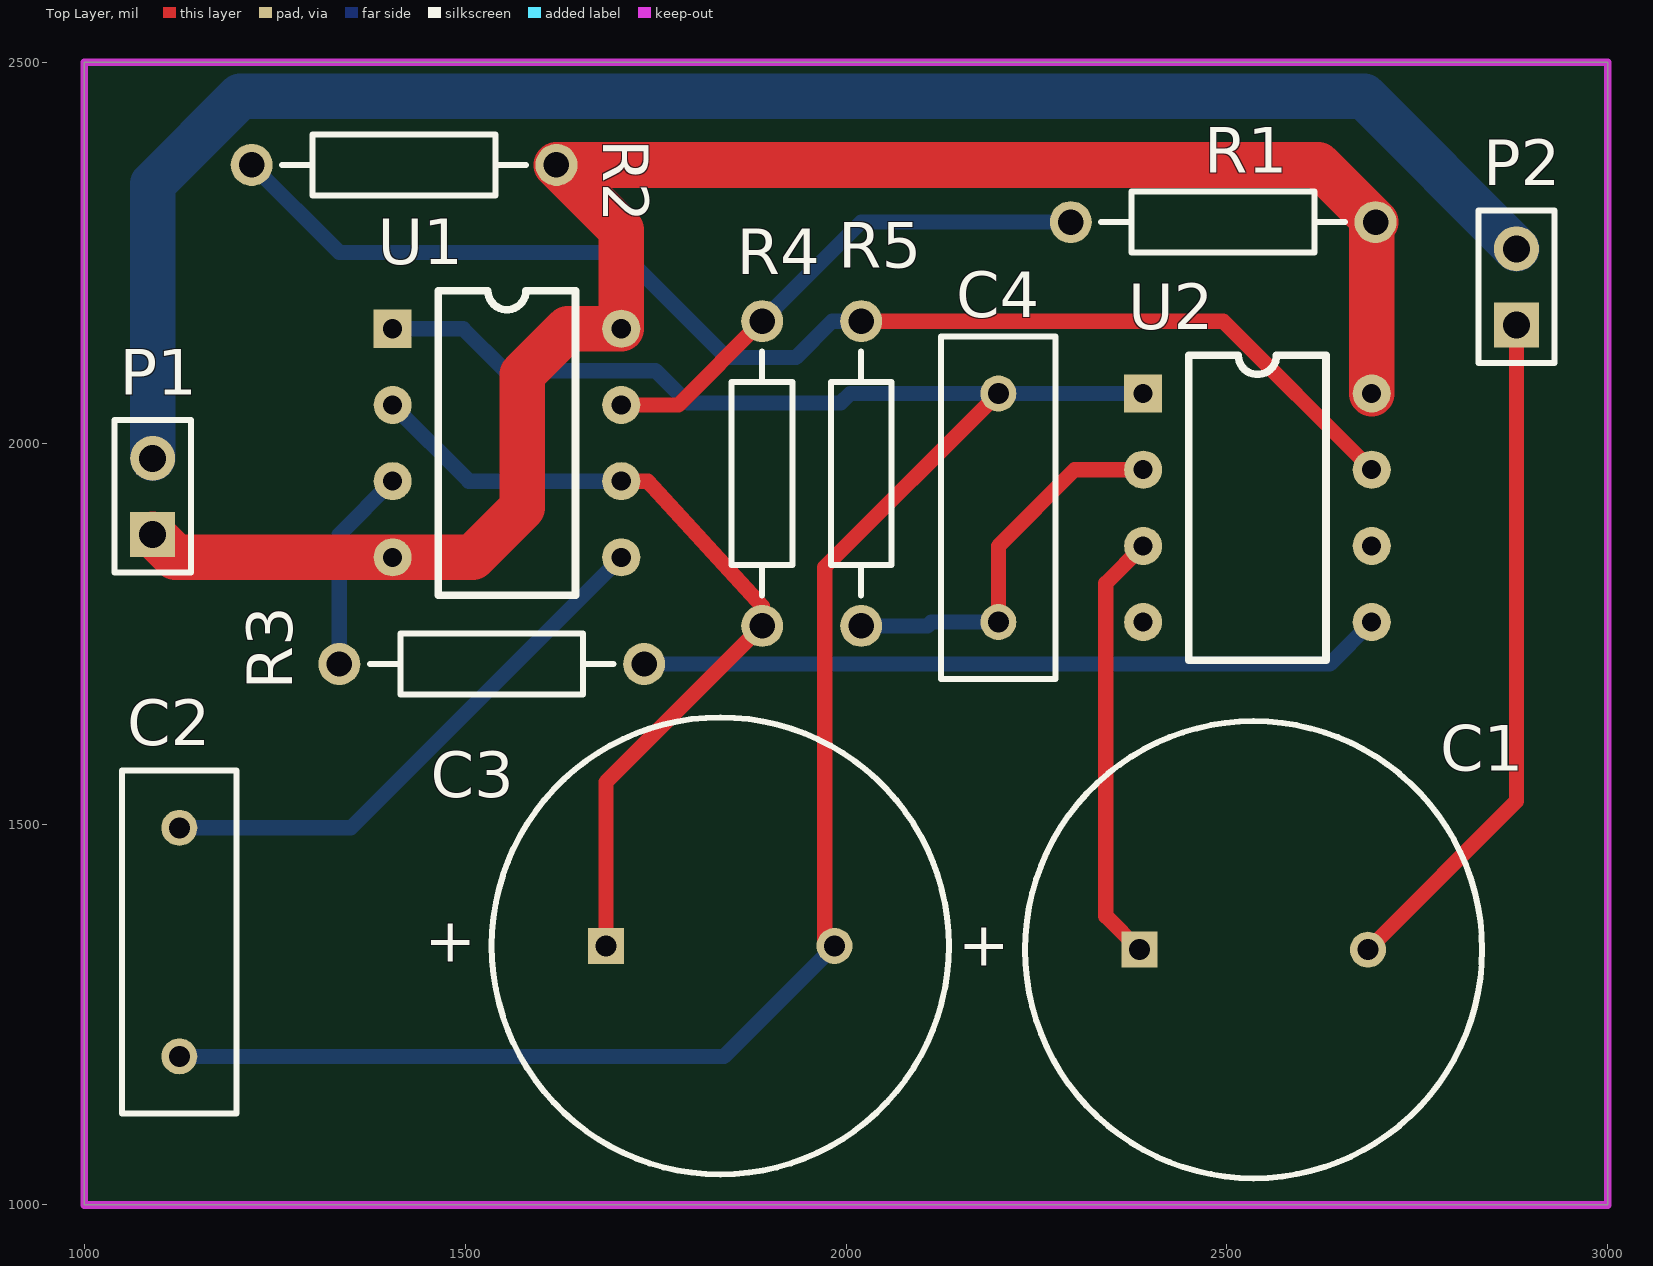
[diagram p0: Top Layer view]
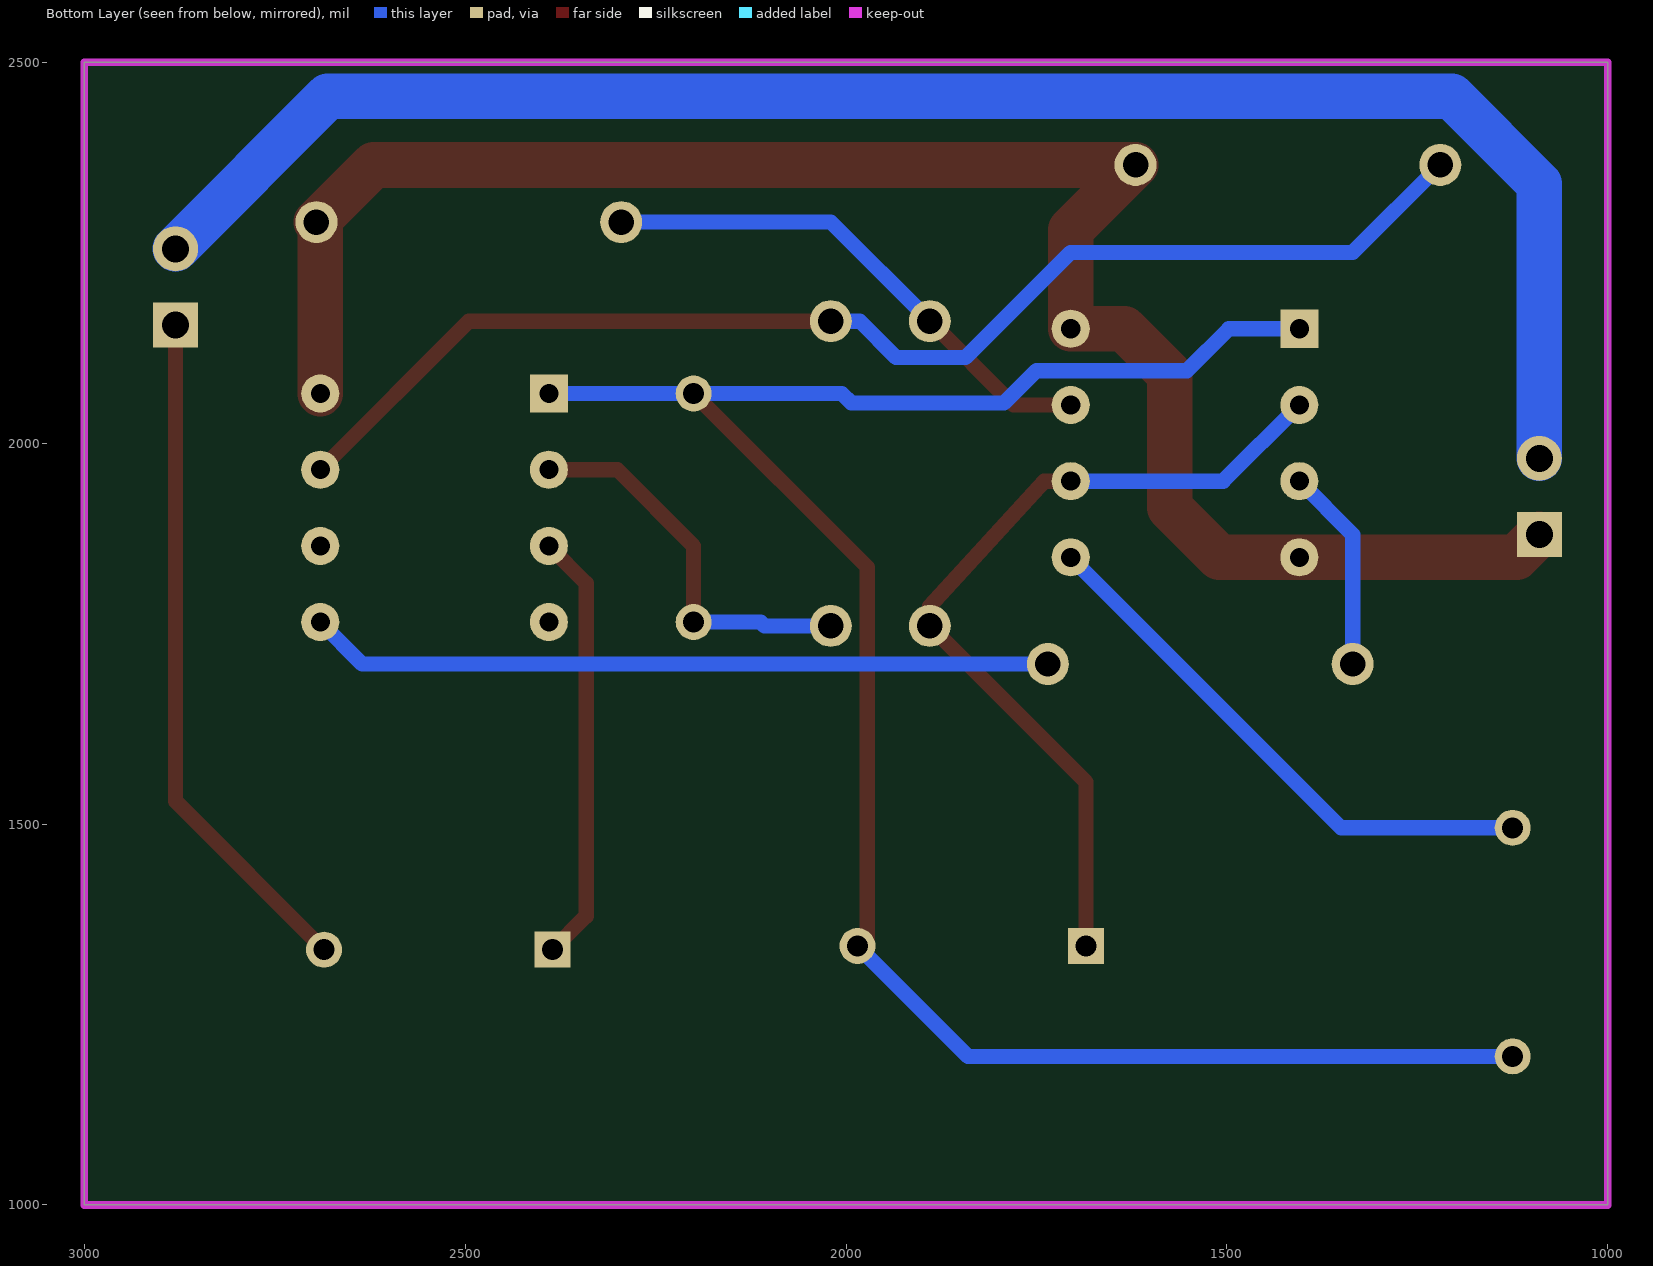
[diagram p1: Bottom Layer view, seen from below]
# Altium PCB MISC80651.PcbDoc
Units mil, origin at the board's own origin, x right, y up, seen from the top; angles counter-clockwise.
Board outline 2000 x 1500 mil, 2 copper layers (Top Layer, Bottom Layer); 13 components, 12 nets, 38 pads, 0 vias.

## Layer stack, top to bottom (the 12.6 mil dielectric is the usual default, probably not edited)
Top Solder: solder mask 0.4, Solder Resist, Dk 3.5
Top Layer: signal copper 1.4
Dielectric 1: dielectric 12.6, FR-4, Dk 4.8
Bottom Layer: signal copper 1.4
Bottom Solder: solder mask 0.4, Solder Resist, Dk 3.5

## Board outline
1000,1000 1000,2500 3000,2500 3000,1000

## Design rules (kind name [scope] priority, off if disabled: settings)
Clearance [All] p1: gap=10
PolygonConnect [All] p1: connectstyle=Relief reliefconductorwidth=10 reliefentries=4 polygonreliefangle="90 Angle" airgapwidth=10
RoutingVias [All] p1: holewidth=28 width=50 viastyle="Through Hole" minholewidth=28 minwidth=50 maxholewidth=28 maxwidth=50
SolderMaskExpansion [All] p1: expansion=4
Width [All] p1: maxlimit=60 minlimit=20 preferedwidth=20
Width GND [InNet('GND')] p2: maxlimit=60 minlimit=60 preferedwidth=60
Width VCC [InNet('VCC')] p3: maxlimit=60 minlimit=60 preferedwidth=60
30 further rules are at their usual default settings.

## Components (designator, comment, footprint, x,y, rotation, side; value= is the part's Value field where it differs from the comment)
C1 "Cap Pol1" RB7.6-15 2535,1335 r180 top
C2 "Cap" RAD-0.3 1125,1345 r90 top
C3 "Cap Pol1" RB7.6-15 1835,1340 r180 top
C4 "Cap" RAD-0.3 2200,1915 r270 top
P1 "Header 2" HDR1X2 1090,1880 r90 top
P2 "Header 2" HDR1X2 2880,2155 r90 top
R1 "Res2" AXIAL-0.4 2495,2290 r0 top
R2 "Res2" AXIAL-0.4 1420,2365 r0 top
R3 "Res2" AXIAL-0.4 1535,1710 r180 top
R4 "Res2" AXIAL-0.4 1890,1960 r90 top
R5 "Res2" AXIAL-0.4 2020,1960 r270 top
U1 "NE555" DIP8 1405,2150 r0 top
U2 "NE555" DIP8 2390,2065 r0 top

## Footprints (in the part's own frame and the unit in brackets; to place one, negate y for a bottom-side part, rotate by r counter-clockwise, add the part's x,y. Pads: shape width x height; smd on the part's side, far side on the other; paste and mask are expansions set on the pad)
AXIAL-0.4 [mm] "Axial Device, Thru-Hole; 2 Leads; 0.4 in Pin Spacing"
  round 1.4 hole 0.85: 1(-5.08,0) 2(5.08,0)
  silkscreen extent -4.06,-1.02 4.06,1.02
DIP8 [mil]
  rect 50x50 hole 25: 1(0,0)
  round 50 hole 25: 2(0,-100) 3(0,-200) 4(0,-300) 5(300,-300) 6(300,-200) 7(300,-100) 8(300,0)
  silkscreen extent 60,-350 240,50
HDR1X2 [mm] "Connector; Header; 2 Position"
  rect 1.5x1.5 hole 0.9: 1(0,0)
  round 1.5 hole 0.9: 2(2.54,0)
  silkscreen extent -1.27,-1.27 3.81,1.27
RAD-0.3 [mm] "Radial Cap, Thru-Hole; 2 Leads; 0.3 in Pin Spacing"
  round 1.2 hole 0.7: 1(-3.81,0) 2(3.81,0)
  silkscreen extent -5.71,-1.91 5.71,1.91
RB7.6-15 [mm] "Polarized Capacitor (Radial); 2 Leads"
  rect 1.2x1.2 hole 0.7: 1(3.81,0)
  round 1.2 hole 0.7: 2(-3.81,0)
  silkscreen extent -7.62,-7.62 7.62,7.62

## Part data
C1 C3: "Polarized Capacitor (Radial)"
C2 C4: "Capacitor"
P1 P2: "Header, 2-Pin"
R1 R2 R3 R4 R5: "Resistor"

## Nets (pads, with @x,y where several pads share a name; then routed paths per layer and width w, separated by ;. In a path a pad name is that pad's centre, name@x,y a point inside that pad or via, vN(x,y) a via of type N, cw(c..) or ccw(c..) an arc to the next point about the centre after c; other vN are vias at no path point)
GND: P1.2 P2.2 | length 2280.5
  Bottom Layer w60: P1.2 1090,2340 1205,2455 2680,2455 P2.2
NetC1_1: C1.1 U2.3 | length 568.5
  Top Layer w20: C1.1 2341,1379 2341,1816 U2.3
NetC2_1: C2.1 C3.2 C4.1 U1.1 U2.1 | length 2783.1
  Top Layer w20: C3.2 1972,1340 1972,1837 C4.1
  Bottom Layer w20: C2.1 1840,1195 C3.2 ; U1.1 1497.5,2150 1552.5,2095 1750,2095 1792.56,2052.44 1993,2052.44 2005.56,2065 C4.1 U2.1
NetC2_2: C2.2 U1.5 | length 727
  Bottom Layer w20: C2.2 1350,1495 U1.5
NetC3_1: C3.1 R4.1 U1.2 U1.6 | length 1129.6
  Top Layer w20: C3.1 1685,1555 R4.1 1890,1786 1740,1950 U1.6
  Bottom Layer w20: U1.2 1505,1950 U1.6
NetC4_2: C4.2 R5.2 U2.2 | length 513.5
  Top Layer w20: C4.2 2200,1865 2300,1965 U2.2
  Bottom Layer w20: R5.2 2107,1760 2112,1765 C4.2
NetR1_1: R1.1 R4.2 U1.7 | length 689.4
  Top Layer w20: U1.7 1780,2050 R4.2
  Bottom Layer w20: R4.2 2020,2290 R1.1
NetR2_1: R2.1 R5.1 U2.7 | length 1675.1
  Top Layer w20: R5.1 2495,2160 U2.7
  Bottom Layer w20: R2.1 1335,2250 1705.44,2250 1843,2112.44 1934.44,2112.44 1982,2160 R5.1
NetR3_1: R3.1 U2.5 | length 977.8
  Bottom Layer w20: R3.1 2635,1710 U2.5
NetR3_2: R3.2 U1.3 | length 269
  Bottom Layer w20: R3.2 1335,1880 U1.3
VCC: P1.1 R1.2 R2.2 U1.4 U1.8 U2.8 | length 2437.5
  Top Layer w60: P1.1 1120,1850 U1.4 1510,1850 1575,1915 1575,2090 1635,2150 U1.8 1705,2280 R2.2 2620,2365 R1.2 2690,2285 U2.8
VOUT: C1.2 P2.1 | length 900.8
  Top Layer w20: C1.2 2880,1530 P2.1
pads on no net: U2.4 U2.6

## Keep-outs
Keep-Out Layer:
  the board outline again, w10